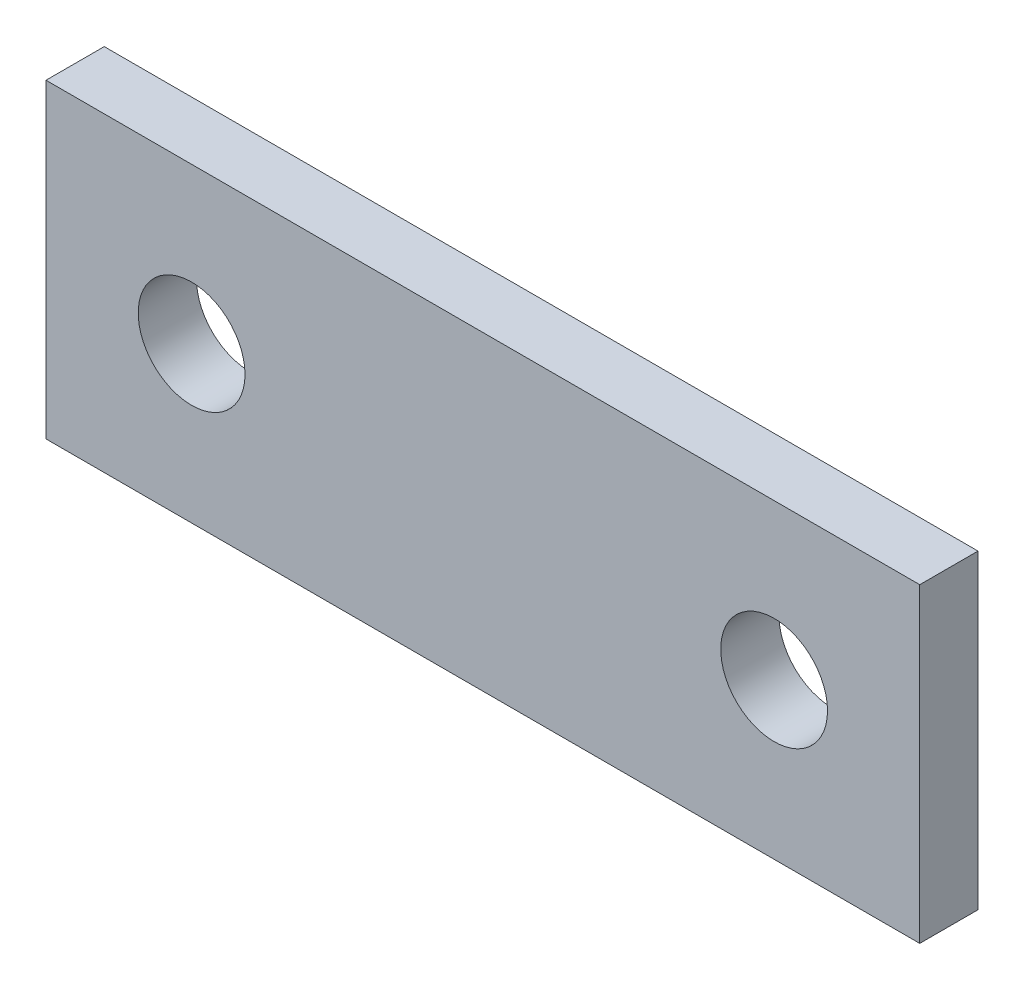
SolidWorks part; units mm, degrees
material "Plain Carbon Steel"
ref_plane "Front Plane" through (0, 0, 0) normal (0, 0, 1) x (1, 0, 0)
ref_plane "Top Plane" through (0, 0, 0) normal (0, 1, 0) x (1, 0, 0)
ref_plane "Right Plane" through (0, 0, 0) normal (1, 0, 0) x (0, 0, -1)
sketch "Sketch1" plane through (0, 0, 0) normal (0, 0, 1) x (1, 0, 0)
  line L1 (0, 0) -> (90, 0)
  line L2 (0, 0) -> (0, -32)
  line L3 (0, -32) -> (90, -32)
  line L4 (90, 0) -> (90, -32)
  point P7 (90, 0)
  point P10 (0, 0)
  dimension "D1" = 90
  dimension "D2" = 32
extrude "Boss-Extrude1" add sketch "Sketch1" along normal blind 6
sketch "Sketch2" plane through (0, 0, 6) normal (0, 0, 1) x (1, 0, 0)
  line L0 (90, 0) -> (0, 0) construction
  line L1 (0, 0) -> (0, -32) construction
  circle A0 centre (15, -16) radius 5.5
  dimension "D3" = 11
  dimension "D1" = 16
  dimension "D2" = 15
extrude "Cut-Extrude1" cut sketch "Sketch2" against normal blind 6
pattern_linear "LPattern1" count 2 spacing 60 along (1, 0, 0) of "Cut-Extrude1"
